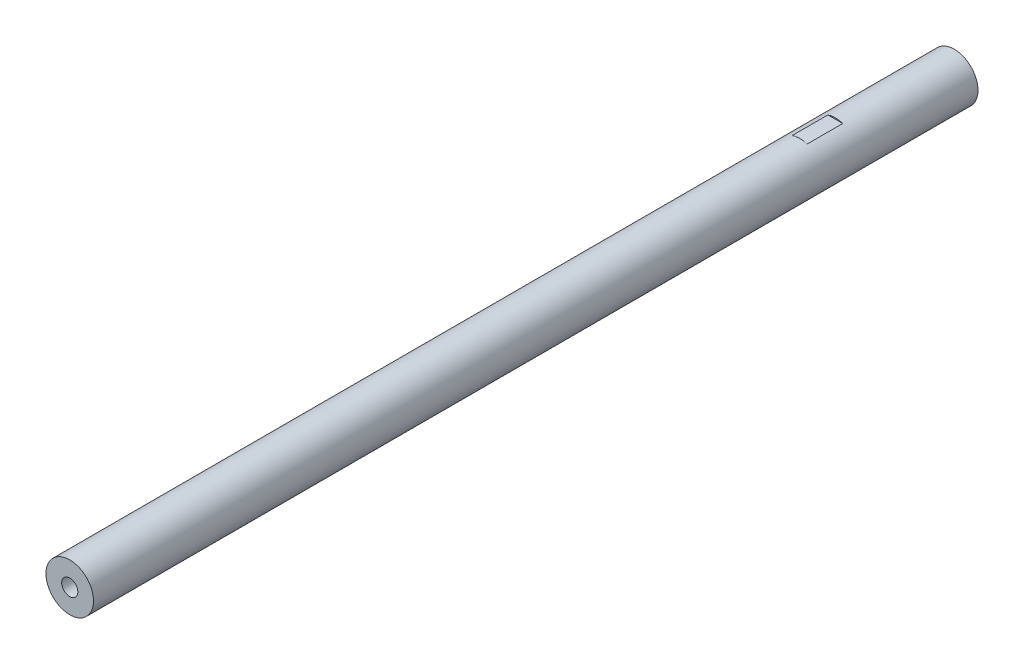
SolidWorks part; units mm, degrees
material "AL6061-T6通用铝"
ref_plane "Front Plane" through (0, 0, 0) normal (0, 0, 1) x (1, 0, 0)
ref_plane "Top Plane" through (0, 0, 0) normal (0, 1, 0) x (1, 0, 0)
ref_plane "Right Plane" through (0, 0, 0) normal (1, 0, 0) x (0, 0, -1)
sketch "Sketch1" plane through (0, 0, 0) normal (0, 0, 1) x (1, 0, 0)
  circle A0 centre (0, 0) radius 10
  dimension "D1" = 20
extrude "Boss-Extrude1" add sketch "Sketch1" along normal mid plane 372
sketch "Sketch2" plane through (0, 0, -186) normal (0, 0, -1) x (-1, 0, 0)
  line L1 (-3.1225, -9.5) -> (3.1225, -9.5)
  line L3 (-3.1225, 9.5) -> (3.1225, 9.5)
  line L5 (-3.1225, -9.5) -> (3.1225, 9.5) construction
  line L6 (-3.1225, 9.5) -> (3.1225, -9.5) construction
  arc A2 (-3.1225, -9.5) -> (3.1225, -9.5) centre (0, 0) ccw
  arc A3 (3.1225, 9.5) -> (-3.1225, 9.5) centre (0, 0) ccw
  dimension "D1" = 20
  dimension "D2" = 19
extrude "Cut-Extrude1" cut sketch "Sketch2" along normal blind 15 from offset 65 offset against normal yes
hole_wizard "M8 Tapped Hole1" positions "Sketch3" profile "Sketch4" tap size "M8" standard "ISO"
sketch "Sketch3" plane through (0, 0, -186) normal (0, 0, -1) x (-1, 0, 0)
  point P0 (0, 0)
cosmetic thread "Cosmetic thread1"
sketch "Sketch4" plane through (0, 0, -186) normal (1, 0, 0) x (0, 1, 0)
  line L0 (0, 0) -> (0, 21.7929)
  line L1 (0, 21.7929) -> (3.4, 19.75)
  line L2 (3.4, 19.75) -> (3.4, 0)
  line L5 (3.4, 0) -> (0, 0)
  line L10 (0, 21.7929) -> (-3.4, 19.75) construction
  line L11 (0, -6.35) -> (0, 107.95) construction
  dimension "螺纹孔钻头直径" = 6.8
  dimension "螺纹孔钻头深度" = 19.75
  dimension "导头角度" = 118
hole_wizard "M8 Tapped Hole2" positions "Sketch5" profile "Sketch6" tap size "M8" standard "ISO"
sketch "Sketch5" plane through (0, 0, 186) normal (0, 0, 1) x (1, 0, 0)
  point P0 (0, 0)
sketch "Sketch6" plane through (0, 0, 186) normal (1, 0, 0) x (0, -1, 0)
  line L0 (0, 0) -> (0, 21.7929)
  line L1 (0, 21.7929) -> (3.4, 19.75)
  line L2 (3.4, 19.75) -> (3.4, 0)
  line L5 (3.4, 0) -> (0, 0)
  line L10 (0, 21.7929) -> (-3.4, 19.75) construction
  line L11 (0, -6.35) -> (0, 107.95) construction
  dimension "螺纹孔钻头直径" = 6.8
  dimension "螺纹孔钻头深度" = 19.75
  dimension "导头角度" = 118
cosmetic thread "Cosmetic thread2" parameters "D1"=16, "D2"=8
